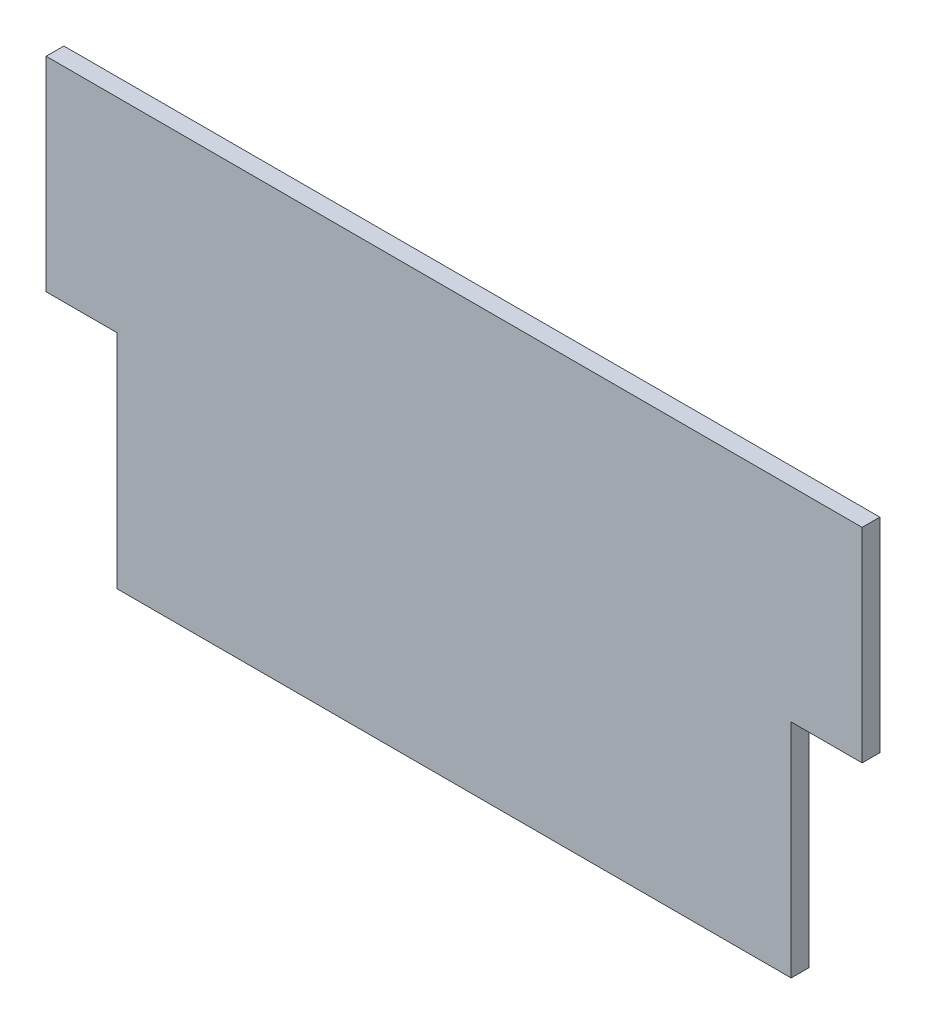
from build123d import *

# Parameters (mm, degrees)
EXTRUDE_1_DEPTH = 10
SKETCH_2_W      = 10
SKETCH_2_H      = 125
EXTRUDE_2_DEPTH = 10
SKETCH_3_W      = 10
SKETCH_3_H      = 125
EXTRUDE_3_DEPTH = 10


with BuildPart() as part:
    # 草图1 → 凸台-拉伸1 (new body)
    with BuildSketch(Plane.XY):
        Polygon((0, 0), (460, 0), (460, -115), (410, -115), (410, -240), (50, -240), (50, -115), (0, -115), align=None)
    extrude(amount=EXTRUDE_1_DEPTH)

    # 草图2 → 凸台-拉伸2 (add)
    with BuildSketch(Plane(origin=(410, 0, 0), x_dir=(0, 0, -1), z_dir=(1, 0, 0))):
        with Locations((-5, -177.5)):
            Rectangle(SKETCH_2_W, SKETCH_2_H)
    extrude(amount=EXTRUDE_2_DEPTH)

    # 草图3 → 凸台-拉伸3 (add)
    with BuildSketch(Plane.ZY.offset(-50)):
        with Locations((5, -177.5)):
            Rectangle(SKETCH_3_W, SKETCH_3_H)
    extrude(amount=EXTRUDE_3_DEPTH)


solid = part.part
